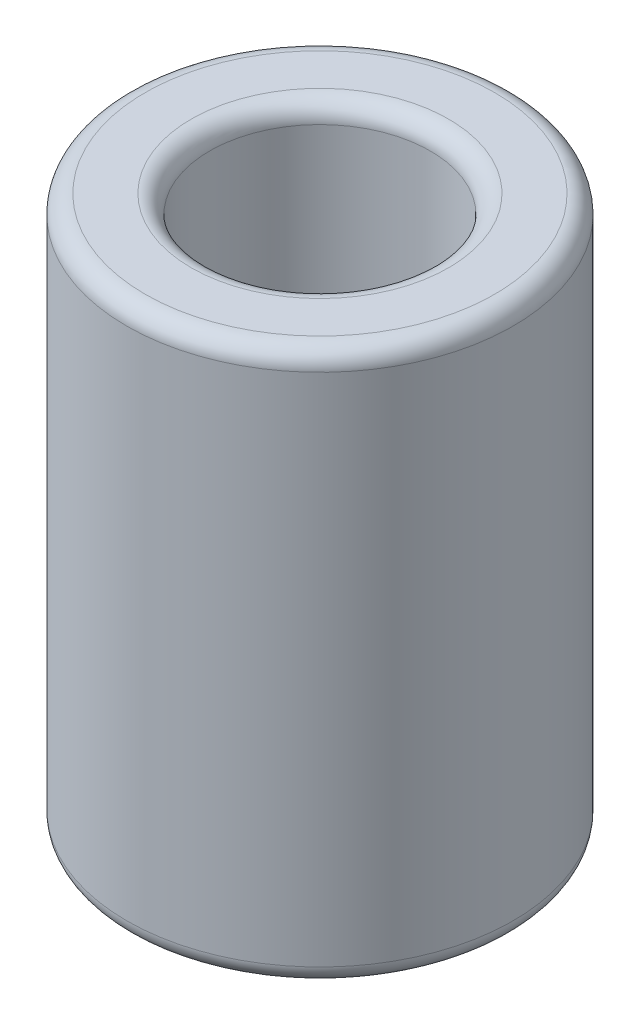
SolidWorks part; units mm, degrees
material "Copper"
ref_plane "Front Plane" through (0, 0, 0) normal (0, 0, 1) x (1, 0, 0)
ref_plane "Top Plane" through (0, 0, 0) normal (0, 1, 0) x (1, 0, 0)
ref_plane "Right Plane" through (0, 0, 0) normal (1, 0, 0) x (0, 0, -1)
sketch "Sketch1" plane through (0, 0, 0) normal (0, 1, 0) x (1, 0, 0)
  circle A0 centre (0, 0) radius 10.5
  circle A1 centre (0, 0) radius 6
  dimension "D1" = 12
  dimension "D2" = 21
extrude "Boss-Extrude1" add sketch "Sketch1" along normal blind 30
fillet "Fillet1" radius 1 4 edges at (0, 0, 6) (0, 30, 6) (0, 0, 10.5) (0, 30, 10.5)
